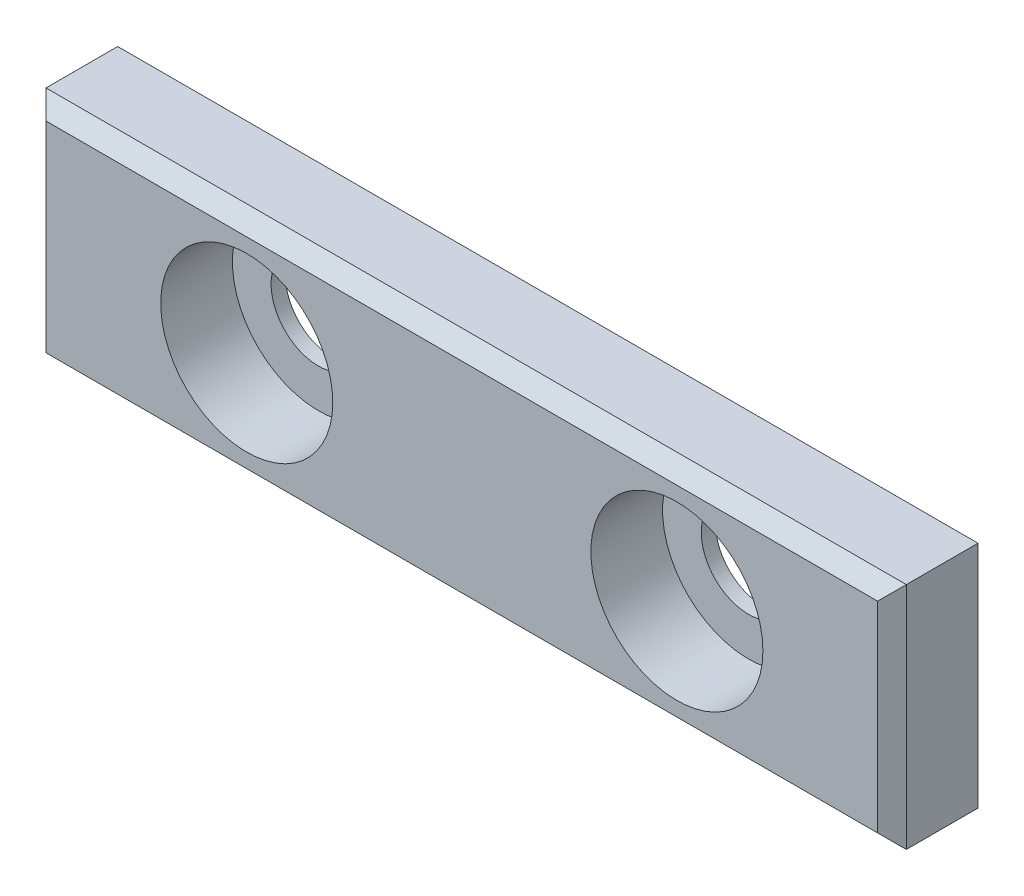
from build123d import *

# Parameters (mm, degrees)
SKETCH1_W          = 60
SKETCH1_H          = 16
BASE_EXTRUDE_DEPTH = 6
SKETCH2_R          = 3.3
CUT_EXTRUDE1_DEPTH = 49.840144417
SKETCH3_R          = 6
CUT_EXTRUDE2_DEPTH = 5
LPATTERN1_COUNT    = 2
LPATTERN1_PITCH    = 30
CHAMFER1_SIZE      = 1


with BuildPart() as part:
    # Sketch1 → Base-Extrude (new body)
    with BuildSketch(Plane.XY):
        with Locations((17.371751412, -2.260451977)):
            Rectangle(SKETCH1_W, SKETCH1_H)
    extrude(amount=BASE_EXTRUDE_DEPTH)

    # Sketch2 → Cut-Extrude1 (cut, through all)
    with BuildSketch(Plane.XY.offset(6)):
        with Locations((2.371751412, -2.260451977)):
            Circle(SKETCH2_R)
    cut_extrude1 = extrude(amount=-CUT_EXTRUDE1_DEPTH, mode=Mode.SUBTRACT)

    # Sketch3 → Cut-Extrude2 (cut)
    with BuildSketch(Plane.XY.offset(6)):
        with Locations((2.371751412, -2.260451977)):
            Circle(SKETCH3_R)
    cut_extrude2 = extrude(amount=-CUT_EXTRUDE2_DEPTH, mode=Mode.SUBTRACT)

    # LPattern1: Cut-Extrude1, Cut-Extrude2 ×2
    with Locations(*[(i * LPATTERN1_PITCH, 0, 0) for i in range(1, LPATTERN1_COUNT)]):
        add(cut_extrude1, mode=Mode.SUBTRACT)
        add(cut_extrude2, mode=Mode.SUBTRACT)

    # Chamfer1
    chamfer1_edges = [part.edges().sort_by_distance(p)[0] for p in [
        (47.371751412, -2.260451977, 6),
        (17.371751412, 5.739548023, 6),
        (-12.628248588, -2.260451977, 6),
        (17.371751412, -10.260451977, 6),
    ]]
    chamfer(chamfer1_edges, length=CHAMFER1_SIZE)


solid = part.part
